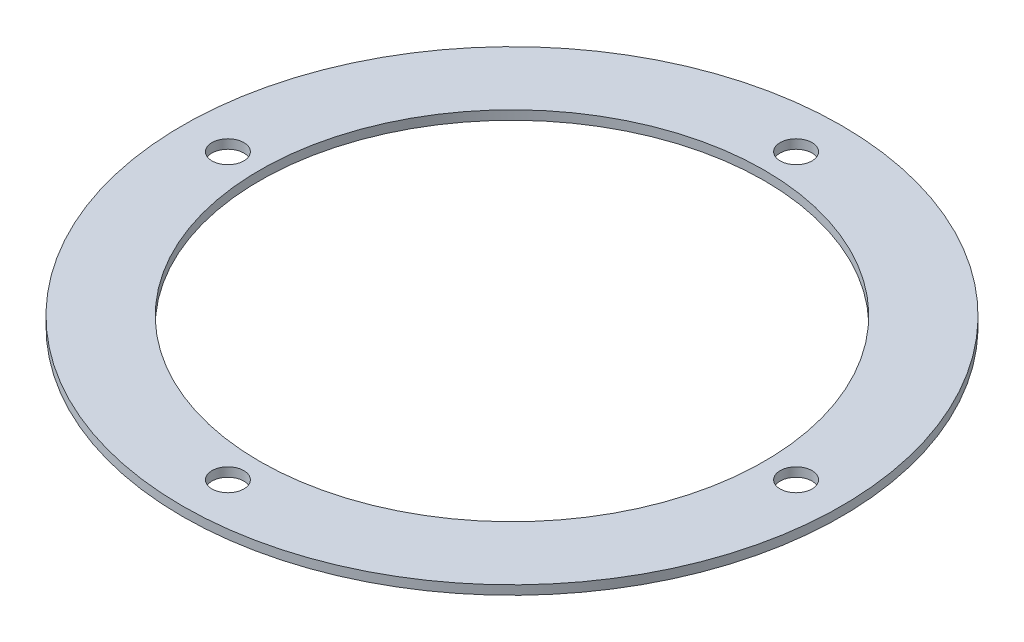
from build123d import *

# Parameters (mm, degrees)
SKETCH1_R           = 72.5
SKETCH1_R_2         = 55.5
BOSS_EXTRUDE1_DEPTH = 2
SKETCH2_R           = 3.5
CUT_EXTRUDE1_DEPTH  = 103.549987811
CIRPATTERN1_COUNT   = 4


with BuildPart() as part:
    # Sketch1 → Boss-Extrude1 (new body)
    with BuildSketch(Plane(origin=(0, 0, 0), x_dir=(1, 0, 0), z_dir=(0, 1, 0))):
        with Locations(Location((0, 0, 0), (0, 0, 270))):
            Circle(SKETCH1_R)
        with Locations(Location((0, 0, 0), (0, 0, 270))):
            Circle(SKETCH1_R_2, mode=Mode.SUBTRACT)
    extrude(amount=BOSS_EXTRUDE1_DEPTH)

    # Sketch2 → Cut-Extrude1 (cut, through all)
    with BuildSketch(Plane(origin=(0, 2, 0), x_dir=(1, 0, 0), z_dir=(0, 1, 0))):
        with Locations(Location((0, 62.5, 0), (0, 0, 270))):
            Circle(SKETCH2_R)
    cut_extrude1 = extrude(amount=-CUT_EXTRUDE1_DEPTH, mode=Mode.SUBTRACT)

    # CirPattern1: Cut-Extrude1 ×4 about axis
    cirpattern1_axis = Axis((0, 0, 0), (0, 1, 0))
    for i in range(1, CIRPATTERN1_COUNT):
        add(cut_extrude1.rotate(cirpattern1_axis, i * 360 / CIRPATTERN1_COUNT), mode=Mode.SUBTRACT)


solid = part.part
